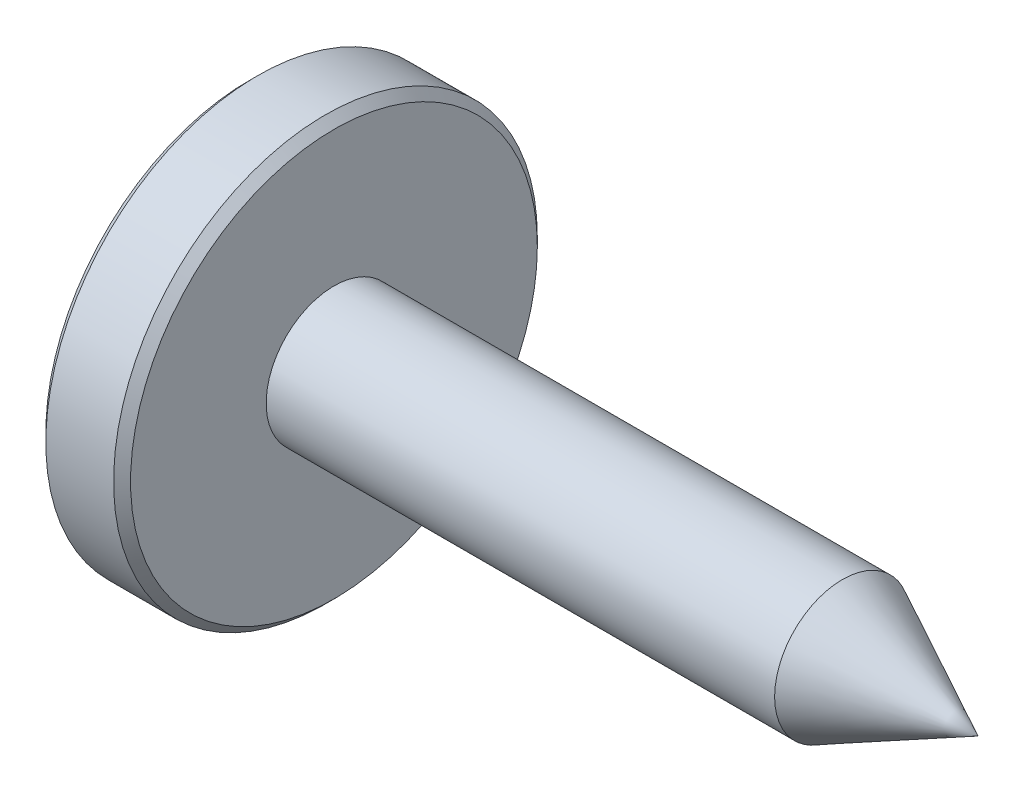
SolidWorks part; units mm, degrees
ref_plane "前视基准面" through (0, 0, 0) normal (0, 0, 1) x (1, 0, 0)
ref_plane "上视基准面" through (0, 0, 0) normal (0, 1, 0) x (1, 0, 0)
ref_plane "右视基准面" through (0, 0, 0) normal (1, 0, 0) x (0, 0, -1)
sketch "草图1" plane through (0, 0, 0) normal (1, 0, 0) x (0, 0, -1)
  circle A0 centre (0, 0) radius 25
  dimension "D1" = 50
extrude "凸台-拉伸1" add sketch "草图1" along normal blind 10
sketch "草图2" plane through (10, 0, 0) normal (1, 0, 0) x (0, 0, -1)
  circle A0 centre (0, 0) radius 8
  dimension "D1" = 16
extrude "凸台-拉伸2" add sketch "草图2" along normal blind 60
cosmetic thread "装饰螺纹线1" parameters "D2"=15
sketch "草图3" plane through (0, 0, 0) normal (0, 0, 1) x (1, 0, 0)
  line L0 (0, 0) -> (95.7683, 0) construction
  line L1 (70, 8) -> (86, 0)
  line L2 (86, 0) -> (70, 0)
  line L3 (70, -8) -> (70, 8) construction
  line L4 (70, 0) -> (70, 8)
  dimension "D1" = 16
revolve "旋转1" add sketch "草图3" angle 360 about L0
chamfer "倒角1" distance 1 angle 45 2 edges at (10, 0, -25) (0, 0, -25)
